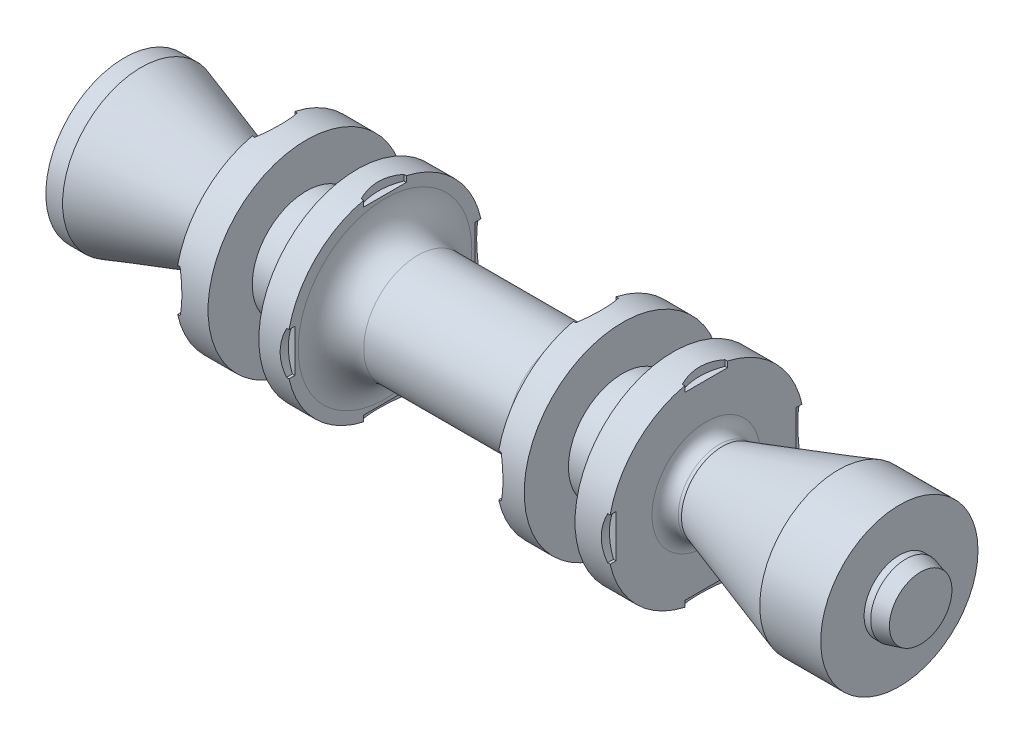
SolidWorks part; units mm, degrees
material "普通碳钢"
ref_plane "Front View" through (0, 0, 0) normal (0, 0, 1) x (1, 0, 0)
ref_plane "Top View" through (0, 0, 0) normal (0, 1, 0) x (1, 0, 0)
ref_plane "Right View" through (0, 0, 0) normal (1, 0, 0) x (0, 0, -1)
sketch "Sketch1" plane through (0, 0, 0) normal (0, 0, 1) x (1, 0, 0)
  line L0 (0, 0) -> (-58.2786, 0) construction
  line L1 (0, 0) -> (0, 31.2509) construction
  line L2 (0, 0) -> (0, 2.15)
  line L3 (0, 2.15) -> (-1.3, 2.15)
  line L4 (-1.3, 2.15) -> (-1.3, 4.8)
  line L5 (-1.3, 4.8) -> (-5.0213, 4.8)
  line L6 (-5.0213, 4.8) -> (-12.1, 2.5)
  line L7 (-12.1, 2.5) -> (-13.1, 2.5)
  line L8 (-13.1, 2.5) -> (-13.1, 6)
  line L9 (-13.1, 6) -> (-15.1, 6)
  line L10 (-15.1, 6) -> (-15.1, 3.3)
  line L11 (-15.1, 3.3) -> (-18.2, 3.3)
  line L12 (-18.2, 3.3) -> (-18.2, 6)
  line L13 (-18.2, 6) -> (-19.9, 6)
  line L14 (-19.9, 6) -> (-19.9, 3.3)
  line L15 (-19.9, 3.3) -> (-32.7, 3.3)
  line L16 (-32.7, 3.3) -> (-32.7, 6)
  line L17 (-32.7, 6) -> (-34.4, 6)
  line L18 (-34.4, 6) -> (-34.4, 3.3)
  line L19 (-34.4, 3.3) -> (-37.5, 3.3)
  line L20 (-37.5, 3.3) -> (-37.5, 6)
  line L21 (-37.5, 6) -> (-39.5, 6)
  line L22 (-39.5, 6) -> (-39.5, 2.5)
  line L23 (-39.5, 2.5) -> (-40.5, 2.5)
  line L24 (-40.5, 2.5) -> (-47.5787, 4.8)
  line L25 (-47.5787, 4.8) -> (-48.6, 4.8)
  line L26 (-48.6, 4.8) -> (-48.6, 2.2)
  line L27 (-48.6, 2.2) -> (-49.9, 2.2)
  line L28 (-49.9, 2.2) -> (-49.9, 0)
  line L29 (-49.9, 0) -> (0, 0)
  point P37 (0, 1.075)
  dimension "D1" = 9.6
  dimension "D2" = 4.3
  dimension "D3" = 1.3
  dimension "D4" = 3.1
  dimension "D5" = 1.7
  dimension "D6" = 2
  dimension "D7" = 13.8
  dimension "D8" = 1.7
  dimension "D9" = 2
  dimension "D10" = 18.6
  dimension "D11" = 18
  dimension "D12" = 12
  dimension "D13" = 9.6
  dimension "D14" = 1.3
  dimension "D15" = 4.4
  dimension "D16" = 38.2
  dimension "D17" = 6.6
  dimension "D18" = 49.9
  dimension "D19" = 1
  dimension "D21" = 1
  dimension "D22" = 2.5
  dimension "D23" = 18
revolve "Revolve1" add sketch "Sketch1" angle 360 about L0
fillet "Fillet1" radius 0.8 2 edges at (-39.5, 0, -2.5) (-13.1, 0, -2.5)
fillet "Fillet3" radius 2 2 edges at (-19.9, 0, -3.3) (-32.7, 0, -3.3)
chamfer "Chamfer1" distance 0.9 angle 15 2 edges at (0, 0, -2.15) (-49.9, 0, -2.2)
sketch "Sketch2" plane through (0, 0, 0) normal (0, 1, 0) x (1, 0, 0)
  line L0 (-39.5, 6) -> (-39.5, -6) construction
  line L1 (-39.5, 1.3) -> (-39.35, 1.3)
  line L2 (-39.5, 1.3) -> (-39.5, -1.3)
  line L3 (-39.5, -1.3) -> (-39.35, -1.3)
  line L5 (-32.7, -6) -> (-32.7, 6) construction
  line L6 (-32.7, 1.3) -> (-32.85, 1.3)
  line L7 (-32.7, 1.3) -> (-32.7, -1.3)
  line L8 (-32.7, -1.3) -> (-32.85, -1.3)
  line L10 (-39.5, 0) -> (-42.605, 0) construction
  arc A0 (-39.35, 1.3) -> (-39.35, -1.3) centre (-42.605, 0) cw
  arc A1 (-32.85, 1.3) -> (-32.85, -1.3) centre (-29.595, 0) ccw
  dimension "D1" = 0.4
  dimension "D2" = 0.15
  dimension "D3" = 2.6
extrude "Cut-Extrude1" cut sketch "Sketch2" against normal blind 10 from offset 15.5
ref_plane "Plane1" through (-26.3, 0, 0) normal (1, 0, 0) x (0, 0, -1)
pattern_circular "CirPattern1" count 4 over 360 about axis through (0, 0, 0) along (1, 0, 0) of "Cut-Extrude1"
mirror "Mirror1" about plane through (-26.3, 0, 0) normal (1, 0, 0) of "CirPattern1", "Cut-Extrude1"
